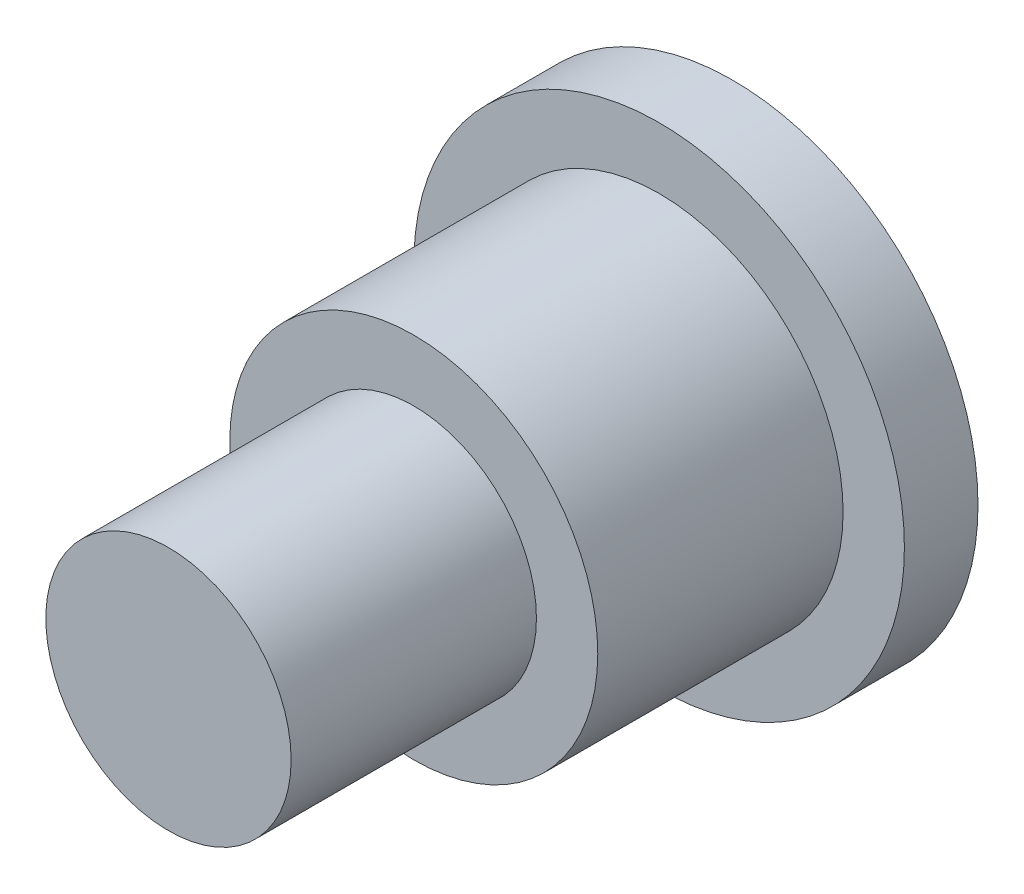
from build123d import *


with BuildPart() as part:
    # Sketch1 → Revolve1 (revolve)
    with BuildSketch(Plane(origin=(0, 0, 0), x_dir=(0, 0, -1), z_dir=(1, 0, 0)), mode=Mode.PRIVATE) as revolve1_sk:
        Polygon((23, 0), (23, 10), (20, 10), (20, 7.5), (10, 7.5), (10, 5), (0, 5), (0, 0), align=None)
    revolve(revolve1_sk.sketch.rotate(Axis((0, 0, 0), (0, 0, -1)), 90), axis=Axis((0, 0, 0), (0, 0, -1)))


solid = part.part
